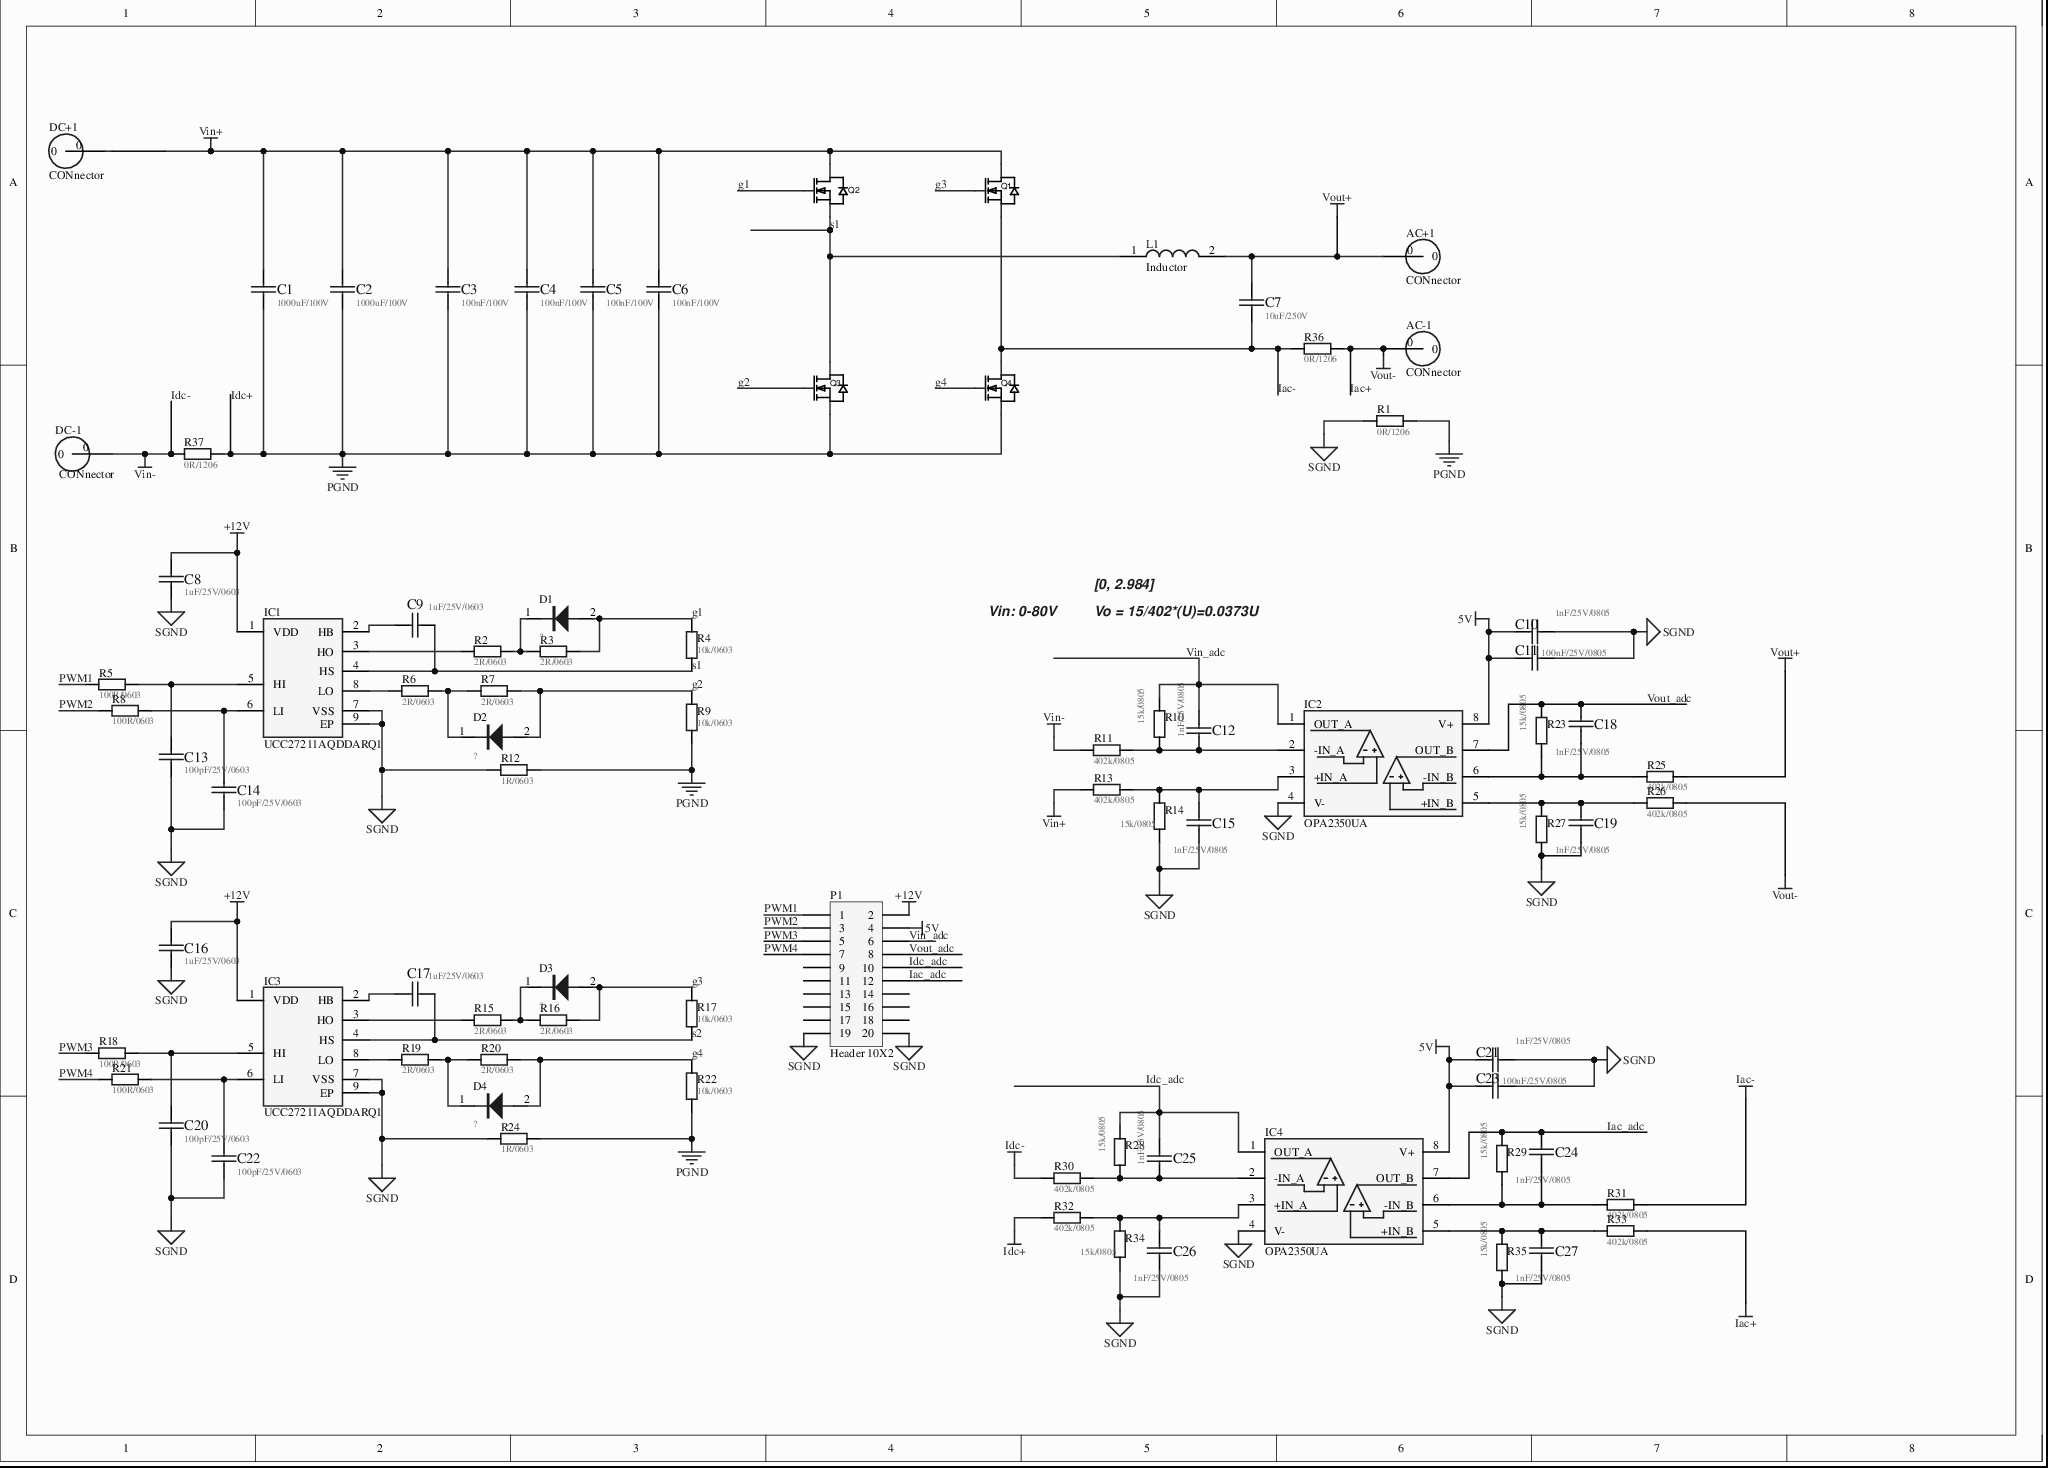
[diagram p0: MISC82254-9.SchDoc]
# Altium project MISC82254-11.PrjPcb
1 sheet, 82 parts. Net scope: global (net labels, ports and power ports of the same name join across sheets).
Board file: MISC82254.PcbDoc

## Sheet MISC82254-9.SchDoc
size A3; SheetNumber: 1; SheetTotal: 1

### Parts
AC+1  CONnector  [CONN-TH_T44001]
AC-1  CONnector  [CONN-TH_T44001]
C1  1000uF/100V  [CAPE]
C2  1000uF/100V  [CAPE]
C3  100nF/100V  [0805C]
C4  100nF/100V  [0805C]
C5  100nF/100V  [0805C]
C6  100nF/100V  [0805C]
C7  10uF/250V  [0805C]
C8  1uF/25V/0603  [0805C]
C9  1uF/25V/0603  [0805C]
C10  1nF/25V/0805  [0805C]
C11  100nF/25V/0805  [0805C]
C12  1nF/25V/0805  [0805C]
C13  100pF/25V/0603  [0805C]
C14  100pF/25V/0603  [0805C]
C15  1nF/25V/0805  [0805C]
C16  1uF/25V/0603  [0805C]
C17  1uF/25V/0603  [0805C]
C18  1nF/25V/0805  [0805C]
C19  1nF/25V/0805  [0805C]
C20  100pF/25V/0603  [0805C]
C21  1nF/25V/0805  [0805C]
C22  100pF/25V/0603  [0805C]
C23  100nF/25V/0805  [0805C]
C24  1nF/25V/0805  [0805C]
C25  1nF/25V/0805  [0805C]
C26  1nF/25V/0805  [0805C]
C27  1nF/25V/0805  [0805C]
D1  ?  [SOD-323]
D2  ?  [SOD-323]
D3  ?  [SOD-323]
D4  ?  [SOD-323]
DC+1  CONnector  [CONN-TH_T44001]
DC-1  CONnector  [CONN-TH_T44001]
IC1  UCC27211AQDDARQ1  [SOIC8 Powerpad]
IC2  OPA2350UA  [SOIC127P600X175-8N]
IC3  UCC27211AQDDARQ1  [SOIC8 Powerpad]
IC4  OPA2350UA  [SOIC127P600X175-8N]
L1  Inductor  [IND-TH_L55.0-W28.0-P20.00-D1.3]
P1  Header 10X2  [HDR2X10]
Q1  IPW60R037CSFD  [TO-247-3_L15.9-W5.1-P5.44-L]  (value not drawn)
Q2  IPW60R037CSFD  [TO-247-3_L15.9-W5.1-P5.44-L]  (value not drawn)
Q3  IPW60R037CSFD  [TO-247-3_L15.9-W5.1-P5.44-L]  (value not drawn)
Q4  IPW60R037CSFD  [TO-247-3_L15.9-W5.1-P5.44-L]  (value not drawn)
R1  0R/1206  [0805R]
R2  2R/0603  [0805R]
R3  2R/0603  [0805R]
R4  10k/0603  [0805R]
R5  100R/0603  [0805R]
R6  2R/0603  [0805R]
R7  2R/0603  [0805R]
R8  100R/0603  [0805R]
R9  10k/0603  [0805R]
R10  15k/0805  [0805R]
R11  402k/0805  [0805R]
R12  1R/0603  [0805R]
R13  402k/0805  [0805R]
R14  15k/0805  [0805R]
R15  2R/0603  [0805R]
R16  2R/0603  [0805R]
R17  10k/0603  [0805R]
R18  100R/0603  [0805R]
R19  2R/0603  [0805R]
R20  2R/0603  [0805R]
R21  100R/0603  [0805R]
R22  10k/0603  [0805R]
R23  15k/0805  [0805R]
R24  1R/0603  [0805R]
R25  402k/0805  [0805R]
R26  402k/0805  [0805R]
R27  15k/0805  [0805R]
R28  15k/0805  [0805R]
R29  15k/0805  [0805R]
R30  402k/0805  [0805R]
R31  402k/0805  [0805R]
R32  402k/0805  [0805R]
R33  402k/0805  [0805R]
R34  15k/0805  [0805R]
R35  15k/0805  [0805R]
R36  0R/1206  [0805R]
R37  0R/1206  [0805R]

### Nets
5V: C10.2 C11.2 C21.2 C23.2 IC2.8(V+) IC4.8(V+) P1.4
+12V: C8.2 C16.2 IC1.1(VDD) IC3.1(VDD) P1.2
Iac+: AC-1.0 R26.2 R33.2 R36.1  [also labelled Vout-]
Iac-: C7.2 Q1.3(S) Q4.2(D) R31.2 R36.2
Idc+: C1.2 C2.2 C3.2 C4.2 C5.2 C6.2 Q3.3(S) Q4.3(S) R1.1 R9.1 R12.2 R22.1 R24.2 R32.1 R37.1  [also labelled PGND]
Idc-: DC-1.0 R11.1 R30.1 R37.2  [also labelled Vin-]
SGND: C8.1 C10.1 C11.1 C13.2 C14.2 C15.2 C16.1 C19.2 C20.2 C21.1 C22.2 C23.1 C26.2 C27.2 IC1.7(VSS) IC1.9(EP) IC2.4(V-) IC3.7(VSS) IC3.9(EP) IC4.4(V-) P1.19 P1.20 R1.2 R12.1 R14.1 R24.1 R27.1 R34.1 R35.1
Vin+: C1.1 C2.1 C3.1 C4.1 C5.1 C6.1 DC+1.0 Q1.2(D) Q2.2(D) R13.1
Vout+: AC+1.0 C7.1 L1.2 R25.2
g1: D1.2(A) Q2.1(G) R3.2 R4.2
g2: D2.2(A) Q3.1(G) R7.2 R9.2
g3: D3.2(A) Q1.1(G) R16.2 R17.2
g4: D4.2(A) Q4.1(G) R20.2 R22.2
Iac_adc: C24.1 IC4.7(OUT_B) P1.12 R29.2
Idc_adc: C25.1 IC4.1(OUT_A) P1.10 R28.2
PWM1: P1.1 R5.1
PWM2: P1.3 R8.1
PWM3: P1.5 R18.1
PWM4: P1.7 R21.1
s1: C9.2 IC1.4(HS) L1.1 Q2.3(S) Q3.2(D) R4.1
s2: C17.2 IC3.4(HS) R17.1
Vin_adc: C12.1 IC2.1(OUT_A) P1.6 R10.2
Vout_adc: C18.1 IC2.7(OUT_B) P1.8 R23.2
NetC9_1: C9.1 IC1.2(HB)
NetC12_2: C12.2 IC2.2(-IN_A) R10.1 R11.2
NetC13_1: C13.1 IC1.5(HI) R5.2
NetC14_1: C14.1 IC1.6(LI) R8.2
NetC15_1: C15.1 IC2.3(+IN_A) R13.2 R14.2
NetC17_1: C17.1 IC3.2(HB)
NetC18_2: C18.2 IC2.6(-IN_B) R23.1 R25.1
NetC19_1: C19.1 IC2.5(+IN_B) R26.1 R27.2
NetC20_1: C20.1 IC3.5(HI) R18.2
NetC22_1: C22.1 IC3.6(LI) R21.2
NetC24_2: C24.2 IC4.6(-IN_B) R29.1 R31.1
NetC25_2: C25.2 IC4.2(-IN_A) R28.1 R30.2
NetC26_1: C26.1 IC4.3(+IN_A) R32.2 R34.2
NetC27_1: C27.1 IC4.5(+IN_B) R33.1 R35.2
NetD1_1: D1.1(K) R2.2 R3.1
NetD2_1: D2.1(K) R6.2 R7.1
NetD3_1: D3.1(K) R15.2 R16.1
NetD4_1: D4.1(K) R19.2 R20.1
NetIC1_3: IC1.3(HO) R2.1
NetIC1_8: IC1.8(LO) R6.1
NetIC3_3: IC3.3(HO) R15.1
NetIC3_8: IC3.8(LO) R19.1

Not connected (* = marked no-connect by the designer): P1 9 11 13 14 15 16 17 18

### Notes on the sheet
- Vin: 0-80V
- Vo = 15/402*(U)=0.0373U
- [0, 2.984]

### Library data of the parts
C1-C27 = CAP
D1-D4 = DIODE_1
IC1 IC3 = UCC27211AQDDARQ1: Integrated Circuit; Manufacturer_Name: Texas Instruments; Datasheet Link: http://www.ti.com/lit/gpn/ucc27211a-q1; Height: 1.7mm; Manufacturer_Part_Number: UCC27211AQDDARQ1; Mouser Part Number: 595-UCC27211AQDDARQ1; Mouser Price/Stock: https://www.mouser.co.uk/ProductDetail/Texas-Instruments/UCC27211AQDDARQ1?qs=n%252BTO0c4TDSYQNOcAHEGCfA%3D%3D; Arrow Part Number: UCC27211AQDDARQ1; Arrow Price/Stock: https://www.arrow.com/en/products/ucc27211aqddarq1/texas-instruments?region=nac
IC2 IC4 = OPA2350UA: Integrated Circuit; Manufacturer_Name: Texas Instruments; Datasheet Link: http://www.ti.com/lit/ds/symlink/opa2350.pdf; Height: 1.75mm; Manufacturer_Part_Number: OPA2350UA; Mouser Part Number: 595-OPA2350UA; Mouser Price/Stock: https://www.mouser.co.uk/ProductDetail/Texas-Instruments/OPA2350UA?qs=7nS3%252BbEUL6t7CV0cQ6bBvg%3D%3D; Arrow Part Number: OPA2350UA; Arrow Price/Stock: https://www.arrow.com/en/products/opa2350ua/texas-instruments?region=nac
L1 = Inductor: Manufacturer_Name: COILCRAFT; Manufacturer_Part_Number: MSS1210-683MED; Datasheet Link: https://www.coilcraft.com/pdfs/MSS1210.pdf; Height: 10.2mm; Mouser Part Number: 994-MSS1210-683MED; Mouser Price/Stock: https://www.mouser.co.uk/ProductDetail/Coilcraft/MSS1210-683MED?qs=zCSbvcPd3pbaONJwG86dvQ%3D%3D
P1 = Header 10X2: Header, 10-Pin, Dual row; LatestRevisionDate: 17-Jul-2002; LatestRevisionNote: Re-released for DXP Platform.; Publisher: Altium Limited
Q1-Q4 = IPW60R037CSFD: Manufacturer: Infineon(英飞凌); Add into BOM: yes; Type: Type N-channel; Drain Source Voltage (Vdss): 650V; Continuous Drain Current (Id): 54A; Power Dissipation (Pd): 245W; Drain Source On Resistance (RDS(on)@Vgs,Id): 37mΩ@10V,32.6A; Gate Threshold Voltage (Vgs(th)@Id): 4.5V@1.63mA; Symbol: IPW60R037CSFD; Device: IPW60R037CSFD; Supplier: LCSC; Supplier Part: C454260; Manufacturer Part: IPW60R037CSFD; JLCPCB Part Class: Extended Part; LCSC Part Name: N沟道 耐压:650V 电流:54A; Supplier Footprint: TO-247-3; Datasheet: https://atta.szlcsc.com/upload/public/pdf/source/20191114/C454260_FF56A5B181A5739A188DE6ACBDAA373C.pdf; Convert to PCB: yes
R1-R37 = Resistor: Value: 1k